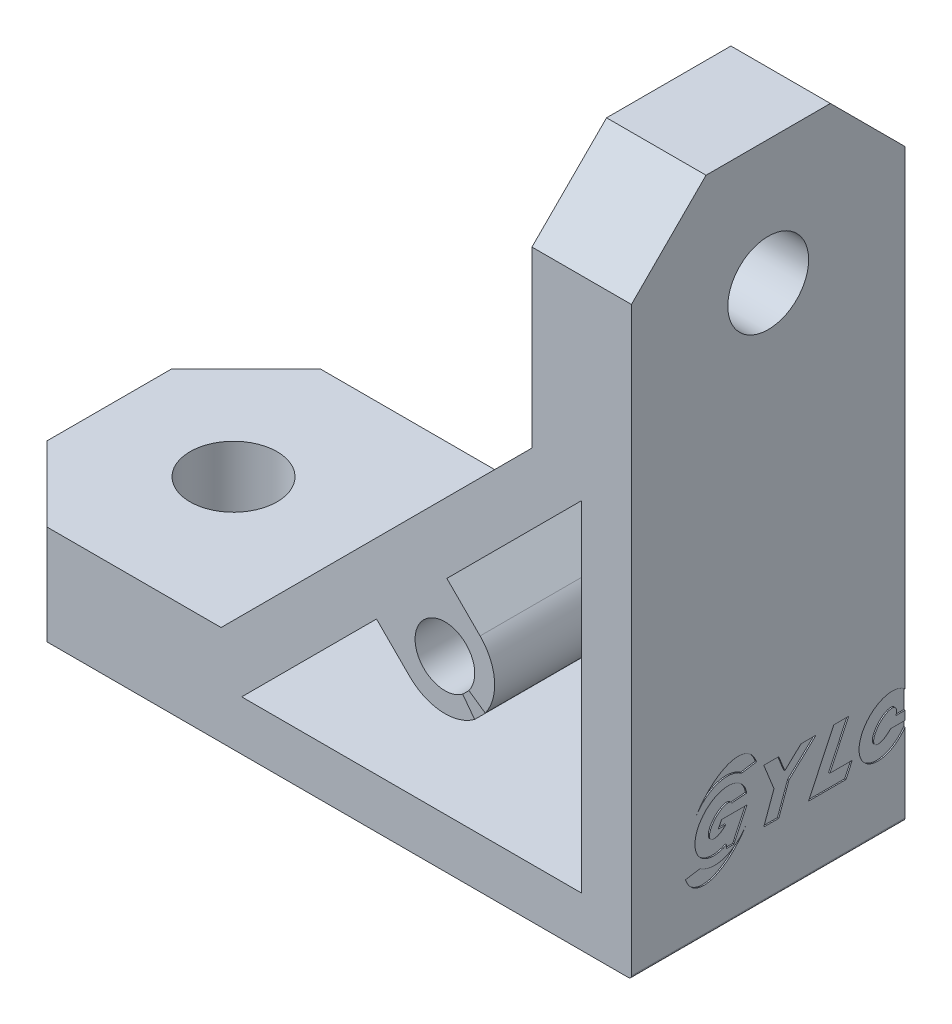
SolidWorks part; units mm, degrees
ref_plane "前视" through (0, 0, 0) normal (0, 0, 1) x (1, 0, 0)
ref_plane "上视" through (0, 0, 0) normal (0, 1, 0) x (1, 0, 0)
ref_plane "右视" through (0, 0, 0) normal (1, 0, 0) x (0, 0, -1)
sketch "Model" plane through (0, 0, 0) normal (0, 0, 1) x (1, 0, 0)
  line L0 (352.7976, 146.5885) -> (380.1407, 146.5885)
  line L1 (366.3123, 154.7601) -> (363.6407, 157.4317)
  line L2 (380.1407, 146.5885) -> (380.1407, 173.9317)
  line L3 (380.1407, 173.9317) -> (369.2976, 163.0885)
  line L4 (371.9691, 160.417) -> (369.2976, 163.0885)
  line L5 (376.1407, 195.5885) -> (384.1407, 195.5885)
  line L6 (331.1407, 150.5885) -> (331.1407, 142.5885)
  line L7 (363.6407, 157.4317) -> (352.7976, 146.5885)
  line L8 (370.5741, 155.6636) -> (371.5298, 154.3804)
  line L9 (335.1407, 146.5885) -> (380.1407, 146.5885) construction
  line L10 (380.1407, 146.5885) -> (380.1407, 191.5885) construction
  line L11 (380.1407, 173.9317) -> (352.7976, 146.5885) construction
  line L12 (376.1407, 175.5885) -> (351.1407, 150.5885)
  line L13 (371.0722, 156.164) -> (372.3859, 155.2501)
  line L22 (351.1407, 150.5885) -> (331.1407, 150.5885)
  line L24 (331.1407, 142.5885) -> (383.9037, 142.5885)
  line L25 (384.1407, 142.8255) -> (384.1407, 195.5885)
  line L27 (376.1407, 195.5885) -> (376.1407, 175.5885)
  line L28 (352.7976, 146.5885) -> (335.1407, 146.5885) construction
  line L29 (380.1407, 191.5885) -> (380.1407, 173.9317) construction
  line L30 (335.1407, 146.5885) -> (335.1407, 146.5885) construction
  line L31 (380.1407, 191.5885) -> (380.1407, 191.5885) construction
  arc A0 (371.0722, 156.164) -> (370.5741, 155.6636) centre (369.1407, 157.5885) ccw
  arc A1 (366.3123, 154.7601) -> (371.5298, 154.3804) centre (369.1407, 157.5885) ccw
  arc A2 (372.3859, 155.2501) -> (371.9691, 160.417) centre (369.1407, 157.5885) ccw
  arc A15 (383.9037, 142.5885) -> (384.1407, 142.8255) centre (383.9037, 142.8255) ccw
  arc A16 (380.1407, 146.5885) -> (380.1407, 146.5885) centre (380.1407, 146.5885) ccw construction
  dimension "D8" = 4.8
  dimension "D10" = 8
  dimension "D1" = 53
  dimension "D2" = 53
  dimension "D3" = 8
  dimension "D4" = 8
  dimension "D5" = 4
  dimension "D6" = 15
  dimension "D7" = 15
  dimension "D9" = 20
  dimension "D11" = 20
extrude "凸台-拉伸1" add sketch "Model" along normal blind 22
sketch "草图1" plane through (0, 142.5885, 0) normal (0, -1, 0) x (-1, 0, 0)
  line L0 (-331.1407, 0) -> (-383.9037, 0) construction
  line L1 (-331.1407, -22) -> (-331.1407, 0) construction
  circle A0 centre (-341.1407, -11) radius 3.5
  circle A3 centre (-341.1407, -41) radius 3.5
  dimension "D1" = 11
  dimension "D2" = 10
  dimension "D3" = 7
  dimension "D6" = 30
extrude "切除-拉伸1" cut sketch "草图1" against normal blind 10
sketch "草图3" plane through (384.1407, 0, 0) normal (1, 0, 0) x (0, 0, -1)
  line L2 (-22, 142.8255) -> (-22, 195.5885) construction
  line L4 (-22, 195.5885) -> (0, 195.5885) construction
  circle A1 centre (-11, 185.5885) radius 3.25
  circle A2 centre (19, 185.5885) radius 3.25
  dimension "D1" = 11
  dimension "D2" = 6.5
  dimension "D3" = 10
  dimension "D5" = 30
extrude "切除-拉伸2" cut sketch "草图3" against normal blind 10
sketch "草图4" plane through (384.1407, 0, 0) normal (1, 0, 0) x (0, 0, -1)
  line L0 (-22, 142.8255) -> (-20.8, 142.8255) construction
  line L1 (-20.8, 142.8255) -> (-19.6, 142.8255) construction
  line L2 (-19.6, 142.8255) -> (-18.4, 142.8255) construction
  line L3 (-18.4, 142.8255) -> (-17.2, 142.8255) construction
  line L4 (-17.2, 142.8255) -> (-16, 142.8255) construction
  line L5 (-16, 142.8255) -> (-14.8, 142.8255) construction
  line L6 (-14.8, 142.8255) -> (-13.6, 142.8255) construction
  line L7 (-22, 142.8255) -> (-22, 141.6255) construction
  line L8 (-22, 141.6255) -> (-22, 140.4255) construction
  line L9 (-22, 140.4255) -> (-22, 139.2255) construction
  line L10 (-22, 142.2255) -> (-19.6, 142.2255) construction
  line L11 (-22, 141.6255) -> (-18.4, 141.6255) construction
  line L12 (-22, 140.4255) -> (-16, 140.4255) construction
  line L13 (-22, 141.0255) -> (-17.2, 141.0255) construction
  line L14 (-22, 139.8255) -> (-14.8, 139.8255) construction
  line L15 (-22, 139.2255) -> (-13.6, 139.2255) construction
  line L16 (-1.6, 150.0255) -> (0.0183, 151.7979) construction
  line L17 (-1.6, 150.0255) -> (-14.8, 150.0255) construction
  line L18 (-1.1569, 149.6209) -> (0.2651, 149.6209)
  line L19 (-1.1569, 149.6209) -> (-1.6, 150.0255) construction
  line L20 (-1.6, 150.0255) -> (-2.9293, 151.2392) construction
  line L21 (-1.6, 150.0255) -> (-2.4091, 149.1393) construction
  line L22 (-19.6, 142.8255) -> (-19.6, 142.2255) construction
  line L23 (-17.2, 142.8255) -> (-17.2, 141.0255) construction
  line L24 (-14.8, 150.0255) -> (-13.1817, 151.7979) construction
  line L25 (-13.9256, 150.8267) -> (-12.7301, 150.9313)
  line L26 (-14.3569, 149.6209) -> (-14.8, 150.0255) construction
  line L27 (-14.8, 150.0255) -> (-16.1293, 151.2392) construction
  line L28 (-14.8, 150.0255) -> (-15.6091, 149.1393) construction
  line L29 (-0.7272, 150.3243) -> (0.4728, 150.3243)
  line L30 (-14.3569, 148.1361) -> (-14.3569, 147.8774)
  line L31 (-14.7414, 150.0897) -> (-12.7134, 150.0897)
  line L32 (-12.7134, 150.0897) -> (-13.7569, 147.8774)
  line L33 (-13.7569, 147.8774) -> (-14.3569, 147.8774)
  line L34 (-14.7414, 150.0897) -> (-15.0175, 149.557)
  line L35 (-15.0175, 149.557) -> (-14.4175, 149.557)
  line L36 (-13.6, 142.8255) -> (-12.4, 142.8255) construction
  line L37 (-12.4, 142.8255) -> (-11.2, 142.8255) construction
  line L38 (-11.2, 142.8255) -> (-10, 142.8255) construction
  line L39 (-22, 139.2255) -> (-22, 138.0255) construction
  line L40 (-22, 138.0255) -> (-8.8, 138.0255) construction
  line L41 (-11.3569, 147.8774) -> (-10.1569, 147.8774)
  line L42 (-11.3569, 147.8774) -> (-10.5361, 150.1327)
  line L43 (-9.3361, 150.1327) -> (-7.1569, 152.1736)
  line L44 (-7.1569, 152.1736) -> (-8.3569, 152.1736)
  line L45 (-8.3569, 152.1736) -> (-9.6644, 150.949)
  line L46 (-9.6644, 150.949) -> (-10.1569, 152.1736)
  line L47 (-10.1569, 152.1736) -> (-11.3569, 152.1736)
  line L48 (-11.3569, 152.1736) -> (-10.5361, 150.1327)
  line L49 (-9.3361, 150.1327) -> (-10.1569, 147.8774)
  line L50 (-11.3569, 147.8774) -> (-13.7569, 147.8774) construction
  line L51 (-5.7304, 152.1736) -> (-7.7569, 147.8774)
  line L52 (-22, 138.6255) -> (-10, 138.6255) construction
  line L53 (-10, 142.8255) -> (-10, 138.6255) construction
  line L54 (-7.7569, 147.8774) -> (-4.7569, 147.8774)
  line L55 (-4.7569, 147.8774) -> (-4.245, 148.9627)
  line L56 (-4.245, 148.9627) -> (-6.045, 148.9627)
  line L57 (-6.045, 148.9627) -> (-4.5304, 152.1736)
  line L58 (-4.5304, 152.1736) -> (-5.7304, 152.1736)
  line L59 (-7.7569, 147.8774) -> (-10.1569, 147.8774) construction
  line L60 (-14.8, 142.8255) -> (-14.8, 139.8255) construction
  line L61 (-8.3569, 152.1736) -> (-10.1569, 152.1736) construction
  line L62 (-13.1307, 152.5159) -> (-11.9452, 152.7016)
  line L63 (-17.6548, 147.3494) -> (-16.4693, 147.5351)
  line L64 (-13.2506, 152.5944) -> (-14.8, 150.0255) construction
  line L65 (-12.7449, 148.786) -> (-14.8, 150.0255) construction
  line L66 (-14.8, 150.0255) -> (-16.9692, 146.429) construction
  line L67 (-12.4, 142.8255) -> (-12.4, 138.6255) construction
  line L68 (-16, 142.8255) -> (-16, 140.4255) construction
  line L69 (-10, 142.8255) -> (-8.8, 142.8255) construction
  line L70 (-22, 142.8255) -> (-22, 150.0255) construction
  line L71 (-22, 150.0255) -> (-14.8, 150.0255) construction
  line L72 (-22, 150.0255) -> (-22, 157.2255) construction
  ellipse E0 centre (-1.6, 150.0255) end of major axis (-2.4091, 149.1393) minor radius 0.6 (-0.7272, 150.3243) -> (-1.1569, 149.6209) ccw
  ellipse E1 centre (-1.6, 150.0255) end of major axis (-3.2183, 148.2531) minor radius 1.8 (0.4728, 150.3243) -> (0.2651, 149.6209) ccw
  ellipse E2 centre (-14.8, 150.0255) end of major axis (-15.6091, 149.1393) minor radius 0.6 (-13.9256, 150.8267) -> (-14.4175, 149.557) ccw
  ellipse E3 centre (-14.8, 150.0255) end of major axis (-16.4183, 148.2531) minor radius 1.8 (-12.7301, 150.9313) -> (-14.3569, 148.1361) ccw
  ellipse E4 centre (-14.8, 150.0255) end of major axis (-16.9692, 146.429) minor radius 2.4 (-11.9452, 152.7016) -> (-16.8551, 151.265) ccw
  ellipse E5 centre (-14.8, 150.0255) end of major axis (-16.3494, 147.4566) minor radius 2.4 (-13.1307, 152.5159) -> (-16.8551, 151.265) ccw
  ellipse E6 centre (-14.8, 150.0255) end of major axis (-16.9692, 146.429) minor radius 2.4 (-17.6548, 147.3494) -> (-12.7449, 148.786) ccw
  ellipse E7 centre (-14.8, 150.0255) end of major axis (-16.3494, 147.4566) minor radius 2.4 (-16.4693, 147.5351) -> (-12.7449, 148.786) ccw
  dimension "D1" = 1.2
  dimension "D2" = 70
  dimension "D3" = 47.602
  dimension "D4" = 11.302
  dimension "D5" = 50
  dimension "D6" = 5
  dimension "D7" = 15
extrude "切除-拉伸3" cut sketch "草图4" against normal blind 0.1
chamfer "倒角2" distance 6 angle 45 4 edges at (380.1407, 195.5885, 22) (331.1407, 146.5885, 22) (331.1407, 146.5885, 0) (380.1407, 195.5885, 0)
